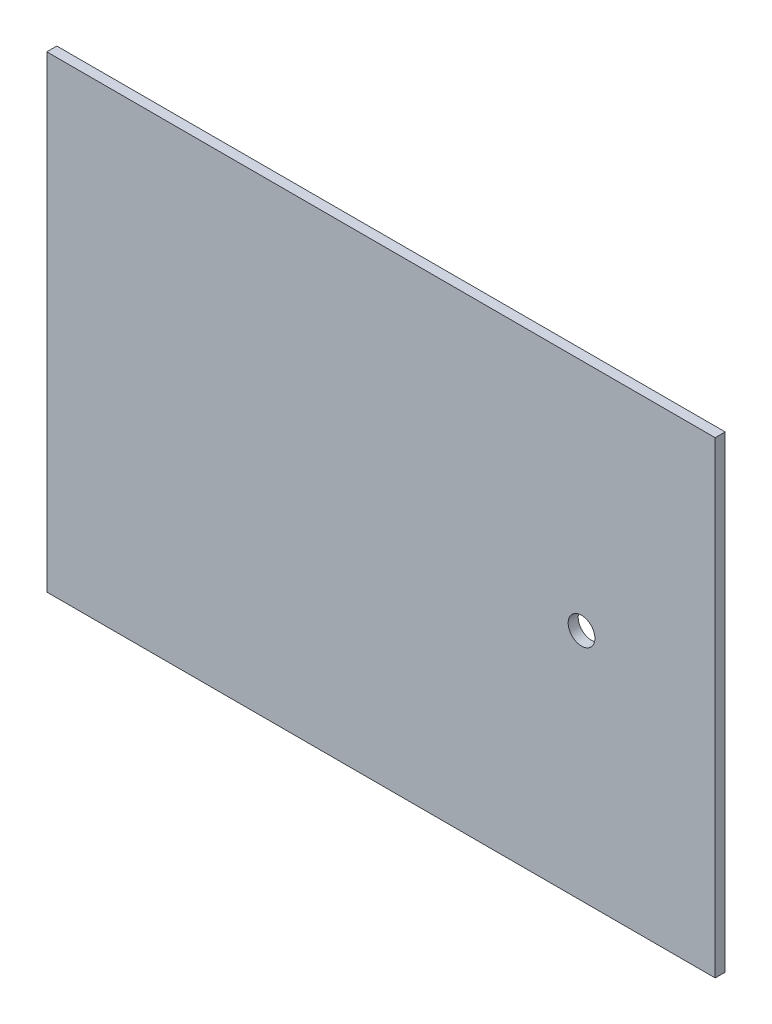
SolidWorks part; units mm, degrees
ref_plane "前视基准面" through (0, 0, 0) normal (0, 0, 1) x (1, 0, 0)
ref_plane "上视基准面" through (0, 0, 0) normal (0, 1, 0) x (1, 0, 0)
ref_plane "右视基准面" through (0, 0, 0) normal (1, 0, 0) x (0, 0, -1)
other "Configuration Table"
sketch "草图1" plane through (0, 0, 0) normal (0, 0, 1) x (1, 0, 0)
  line L0 (-100, -70) -> (100, -70)
  line L1 (100, -70) -> (100, 70)
  line L2 (100, 70) -> (-100, 70)
  line L3 (-100, 70) -> (-100, -70)
  point P0 (0, 0)
  dimension "D1" = 100
  dimension "D2" = 200
  dimension "D3" = 70
  dimension "D4" = 140
extrude "凸台-拉伸1" add sketch "草图1" against normal mid plane 3
sketch "草图2" plane through (0, 0, 0) normal (0, 0, 1) x (1, 0, 0)
  circle A0 centre (60, 0) radius 4
  point P0 (0, 0)
  dimension "D1" = 8
  dimension "D2" = 60
extrude "切除-拉伸1" cut sketch "草图2" against normal mid plane 23
